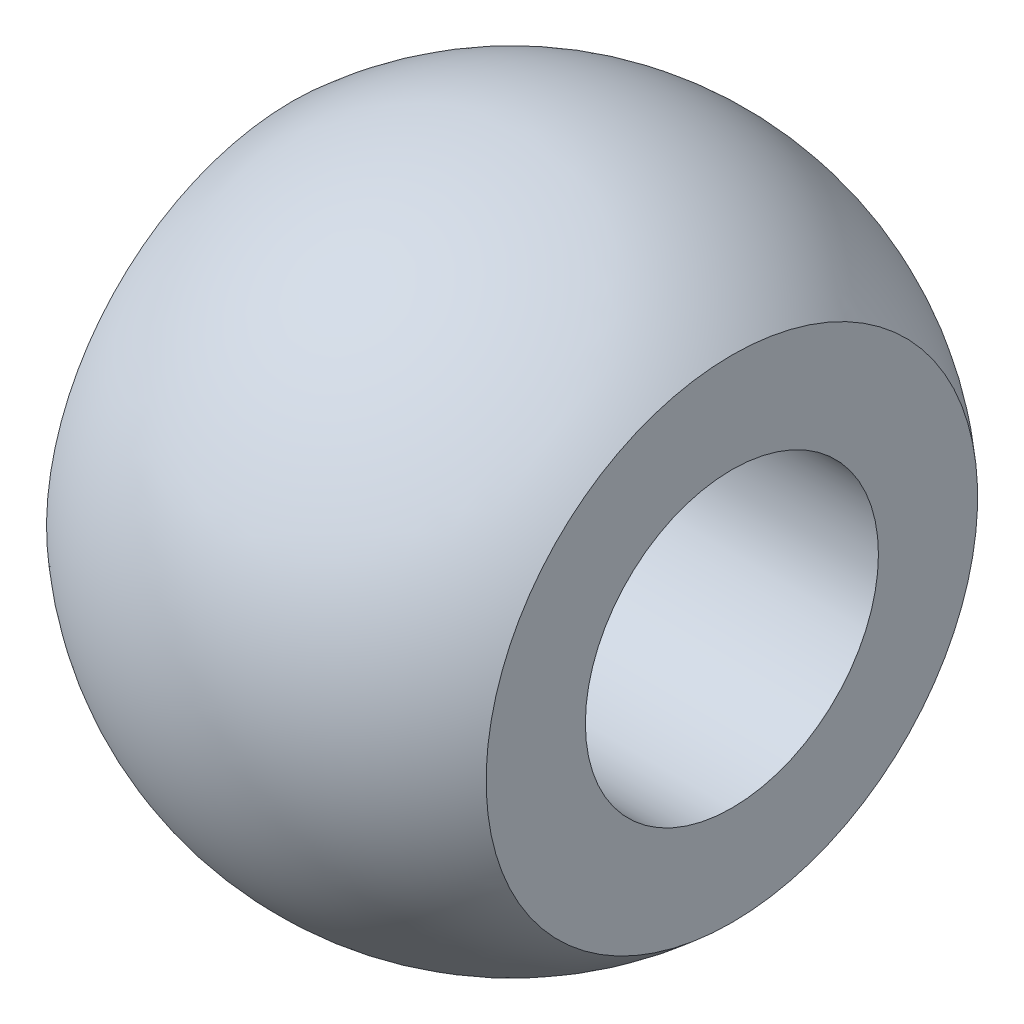
from build123d import *

# Parameters (mm, degrees)
SKETCH4_W          = 4.737450542
SKETCH4_H          = 9.271952016
CUT_EXTRUDE2_DEPTH = 10
SKETCH5_R          = 2
CUT_EXTRUDE3_DEPTH = 20


with BuildPart() as part:
    # Sketch1 → Revolve4 (revolve)
    with BuildSketch(Plane.XY):
        with BuildLine():
            Line((0, 4.5), (0, -4.5))
            ThreePointArc((0, -4.5), (4.5, 0), (0, 4.5))
        make_face()
    revolve(axis=Axis((0, 4.5, 0), (0, -1, 0)))

    # Sketch4 → Cut-Extrude2 (cut, symmetric)
    with BuildSketch(Plane.XY):
        with Locations((5.368725271, -0.018109281)):
            Rectangle(SKETCH4_W, SKETCH4_H)
        with Locations((-5.368725271, -0.018109281)):
            Rectangle(SKETCH4_W, SKETCH4_H)
    extrude(amount=CUT_EXTRUDE2_DEPTH, both=True, mode=Mode.SUBTRACT)

    # Sketch5 → Cut-Extrude3 (cut)
    with BuildSketch(Plane.ZY.offset(3)):
        with Locations(Location((0, 0, 0), (0, 0, 270))):
            Circle(SKETCH5_R)
    extrude(amount=-CUT_EXTRUDE3_DEPTH, mode=Mode.SUBTRACT)


solid = part.part
